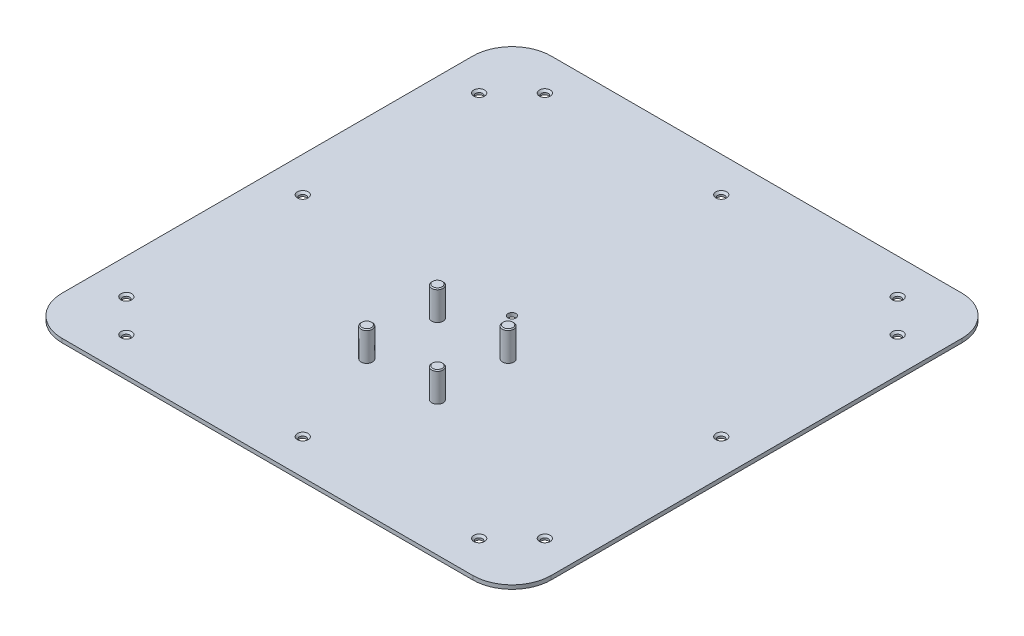
SolidWorks part; units mm, degrees
ref_plane "Front Plane" through (0, 0, 0) normal (0, 0, 1) x (1, 0, 0)
ref_plane "Top Plane" through (0, 0, 0) normal (0, 1, 0) x (1, 0, 0)
ref_plane "Right Plane" through (0, 0, 0) normal (1, 0, 0) x (0, 0, -1)
sketch "Sketch1" plane through (0, 0, 0) normal (0, 1, 0) x (1, 0, 0)
  line L1 (-104.75, -124.75) -> (104.75, -124.75)
  line L2 (-124.75, -104.75) -> (-124.75, 104.75)
  line L3 (-104.75, 124.75) -> (104.75, 124.75)
  line L4 (124.75, -104.75) -> (124.75, 104.75)
  line L5 (-124.75, -124.75) -> (124.75, 124.75) construction
  line L6 (-124.75, 124.75) -> (124.75, -124.75) construction
  arc A0 (124.75, -104.75) -> (104.75, -124.75) centre (104.75, -104.75) cw
  arc A1 (-104.75, -124.75) -> (-124.75, -104.75) centre (-104.75, -104.75) cw
  arc A2 (124.75, 104.75) -> (104.75, 124.75) centre (104.75, 104.75) ccw
  arc A3 (-124.75, 104.75) -> (-104.75, 124.75) centre (-104.75, 104.75) cw
  circle A4 centre (-90, 106.75) radius 1.75
  circle A5 centre (0, 106.75) radius 1.75
  circle A6 centre (90, 106.75) radius 1.75
  circle A7 centre (106.75, 90) radius 1.75
  circle A8 centre (106.75, 0) radius 1.75
  circle A9 centre (106.75, -90) radius 1.75
  circle A10 centre (90, -106.75) radius 1.75
  circle A11 centre (0, -106.75) radius 1.75
  circle A12 centre (-90, -106.75) radius 1.75
  circle A13 centre (-106.75, -90) radius 1.75
  circle A14 centre (-106.75, 0) radius 1.75
  circle A15 centre (-106.75, 90) radius 1.75
  circle A16 centre (0, 0) radius 2
  point P25 (0, 0)
  point P48 (0, 0)
  dimension "D3" = 20
  dimension "D4" = 3.5
  dimension "D6" = 4
  dimension "D1" = 249.5
  dimension "D2" = 249.5
  dimension "D5" = 4
extrude "Boss-Extrude1" add sketch "Sketch1" along normal blind 2
chamfer "Chamfer1" distance 1 angle 45 12 edges at (-106.75, 2, 1.75) (-106.75, 2, 91.75) (-90, 2, 108.5) (0, 2, 108.5) (90, 2, 108.5) (106.75, 2, 91.75) (106.75, 2, 1.75) (106.75, 2, -88.25) (90, 2, -105) (0, 2, -105) (-90, 2, -105) (-106.75, 2, -88.25)
sketch "Sketch2" plane through (0, 2, 0) normal (0, 1, 0) x (1, 0, 0)
  line L1 (-18.0312, -56.0624) -> (18.0312, -56.0624) construction
  line L2 (-18.0312, -56.0624) -> (-18.0312, -20) construction
  line L3 (-18.0312, -20) -> (18.0312, -20) construction
  line L4 (18.0312, -56.0624) -> (18.0312, -20) construction
  line L5 (-18.0312, -56.0624) -> (18.0312, -20) construction
  line L6 (-18.0312, -20) -> (18.0312, -56.0624) construction
  circle A0 centre (0, -38.0312) radius 25.5 construction
  point P0 (0, -38.0312)
  dimension "D1" = 51
  dimension "D2" = 20
sketch "Sketch3" plane through (0, 2, 0) normal (0, 1, 0) x (1, 0, 0)
  circle A0 centre (-18.0312, -20) radius 2.9
  circle A1 centre (18.0312, -20) radius 2.9
  circle A2 centre (18.0312, -56.0624) radius 2.9
  circle A3 centre (-18.0312, -56.0624) radius 2.9
  dimension "D1" = 5.8
extrude "Boss-Extrude2" add sketch "Sketch3" along normal blind 15
chamfer "Chamfer2" distance 0.5 angle 45 4 edges at (-18.0312, 17, 58.9624) (18.0312, 17, 58.9624) (18.0312, 17, 22.9) (-18.0312, 17, 22.9)
